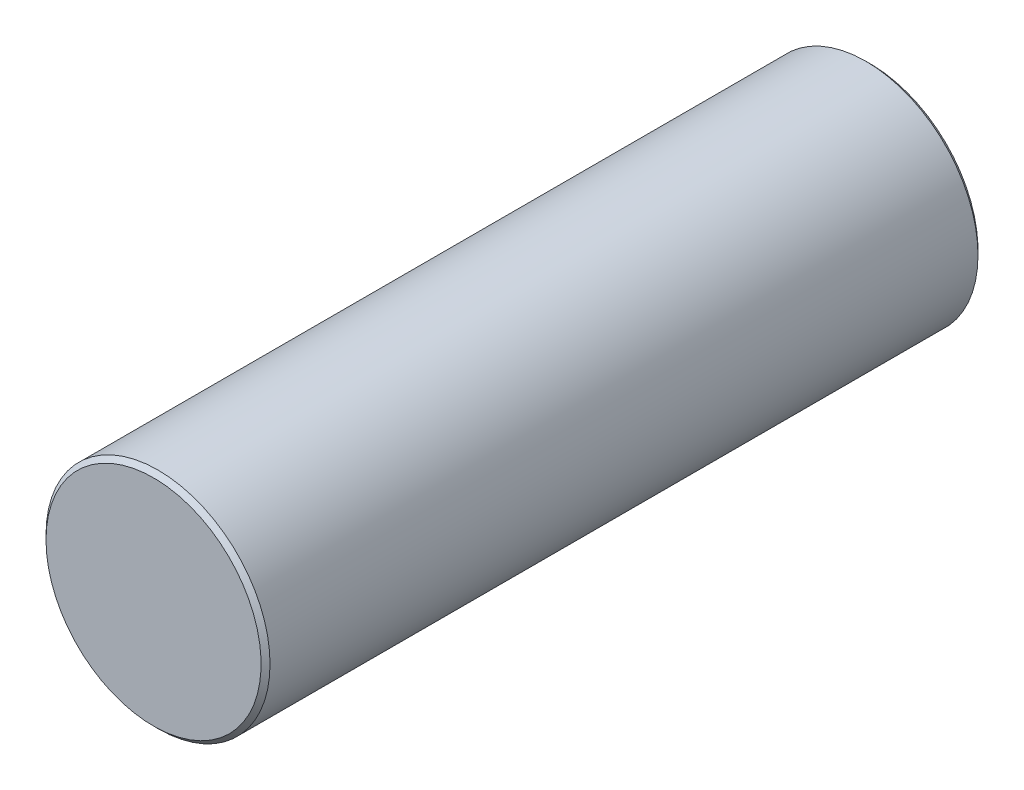
SolidWorks part; units mm, degrees
ref_plane "Front Plane" through (0, 0, 0) normal (0, 0, 1) x (1, 0, 0)
ref_plane "Top Plane" through (0, 0, 0) normal (0, 1, 0) x (1, 0, 0)
ref_plane "Right Plane" through (0, 0, 0) normal (1, 0, 0) x (0, 0, -1)
other "Configuration Table"
ref_plane "Plane1" through (0, 0, 0) normal (0, -1, 0) x (1, 0, 0)
sketch "Sketch1" plane through (0, 0, 0) normal (0, -1, 0) x (1, 0, 0)
  line L0 (12, 80) -> (0, 80)
  line L1 (0, 80) -> (0, 0)
  line L2 (0, 0) -> (12, 0)
  line L3 (12, 0) -> (12.5, 0.5)
  line L4 (12.5, 0.5) -> (12.5, 79.5)
  line L5 (12.5, 79.5) -> (12, 80)
  line L6 (0, 80) -> (0, 0) construction
revolve "Revolve1" add sketch "Sketch1" angle 360 about L6
